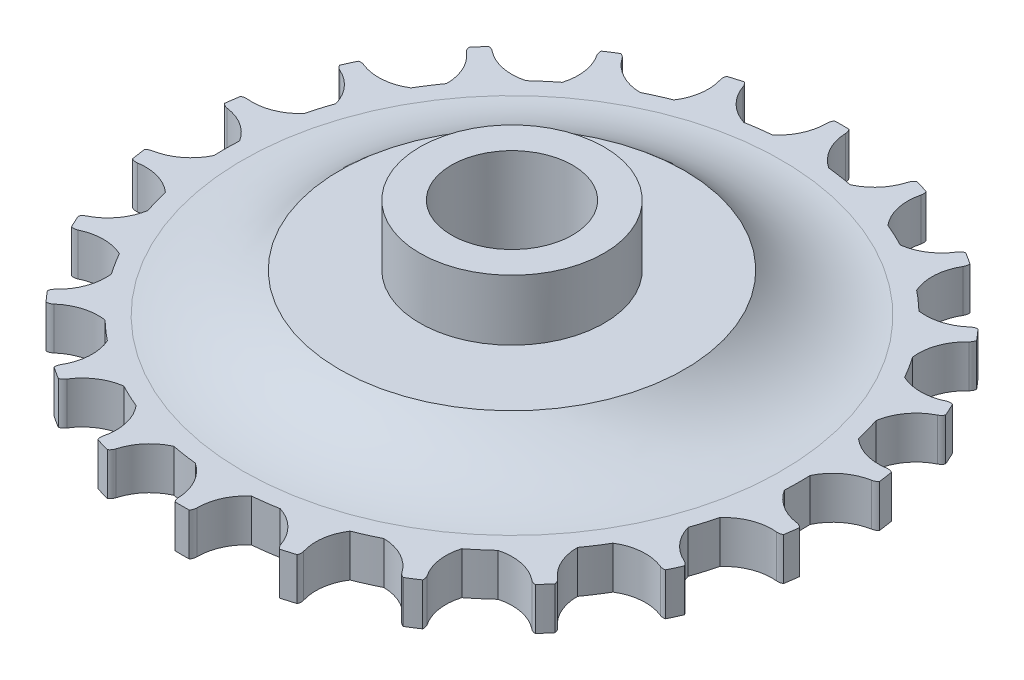
SolidWorks part; units mm, degrees
ref_plane "Front Plane" through (0, 0, 0) normal (0, 0, 1) x (1, 0, 0)
ref_plane "Top Plane" through (0, 0, 0) normal (0, 1, 0) x (1, 0, 0)
ref_plane "Right Plane" through (0, 0, 0) normal (1, 0, 0) x (0, 0, -1)
other "Configuration Table"
sketch "Sketch1" plane through (0, 0, 0) normal (0, 1, 0) x (1, 0, 0)
  line L0 (0, 55) -> (0, 0) construction
  line L1 (-7.2581, 50.4809) -> (0, 0) construction
  line L2 (0, 0) -> (7.2581, 50.4809) construction
  line L3 (-7.2581, 50.4809) -> (7.2581, 50.4809) construction
  circle A62 centre (0, 0) radius 10
  circle A64 centre (0, 0) radius 47.5 construction
  arc A65 (1.4988, 53.5593) -> (-1.4999, 53.4811) centre (0, 53.5) ccw
  arc A66 (-1.4999, 53.4811) -> (-4.294, 47.3055) centre (-9.4992, 53.3805) cw
  arc A67 (1.4988, 53.5593) -> (5.0355, 47.2323) centre (9.4926, 53.8757) ccw
  arc A68 (13.6282, 51.7373) -> (9.2075, 46.5991) centre (5.9246, 53.8944) cw
  arc A69 (16.5275, 50.9675) -> (13.6282, 51.7373) centre (15.0727, 51.3329) ccw
  arc A70 (16.5275, 50.9675) -> (18.1384, 43.9004) centre (24.2866, 49.019) ccw
  arc A71 (27.6523, 45.8021) -> (21.963, 42.1174) centre (20.8684, 50.0422) cw
  arc A72 (30.2172, 44.2466) -> (27.6523, 45.8021) centre (28.9243, 45.0071) ccw
  arc A73 (30.2172, 44.2466) -> (29.7718, 37.012) centre (37.1131, 40.1911) ccw
  arc A74 (39.4361, 36.1562) -> (32.9392, 34.2237) centre (34.1216, 42.1358) cw
  arc A75 (41.459, 33.9412) -> (39.4361, 36.1562) centre (40.4326, 35.035) ccw
  arc A76 (41.459, 33.9412) -> (38.9934, 27.125) centre (46.9329, 28.1071) ccw
  arc A77 (48.0251, 23.5812) -> (41.2468, 23.5574) centre (44.6105, 30.8159) cw
  arc A78 (49.3419, 20.886) -> (48.0251, 23.5812) centre (48.6653, 22.2247) ccw
  arc A79 (49.3419, 20.886) -> (45.0559, 15.0406) centre (52.9504, 13.746) ccw
  arc A80 (52.7233, 9.0958) -> (46.2129, 10.9826) centre (51.4853, 16.9994) cw
  arc A81 (53.2275, 6.1387) -> (52.7233, 9.0958) centre (52.9554, 7.6138) ccw
  arc A82 (53.2275, 6.1387) -> (47.4682, 1.7376) centre (54.6783, -1.7286) ccw
  arc A83 (53.1502, -6.1265) -> (47.4351, -2.482) centre (54.189, 1.8057) cw
  arc A84 (52.8009, -9.1059) -> (53.1502, -6.1265) centre (52.9554, -7.6138) ccw
  arc A85 (52.8009, -9.1059) -> (46.035, -11.7061) centre (51.9764, -17.0633) ccw
  arc A86 (49.2712, -20.8525) -> (44.8144, -15.7455) centre (52.5027, -13.5342) cw
  arc A87 (48.0966, -23.6127) -> (49.2712, -20.8525) centre (48.6653, -22.2247) ccw
  arc A88 (48.0966, -23.6127) -> (40.8722, -24.2015) centre (45.0637, -31.0155) ccw
  arc A89 (41.4006, -33.8892) -> (38.5631, -27.7333) centre (46.563, -27.7777) cw
  arc A90 (39.4959, -36.2066) -> (41.4006, -33.8892) centre (40.4326, -35.035) ccw
  arc A91 (39.4959, -36.2066) -> (32.3983, -34.7362) centre (34.5002, -42.4551) ccw
  arc A92 (30.1759, -44.1803) -> (29.1876, -37.4744) centre (36.8509, -39.7708) cw
  arc A93 (27.6955, -45.8673) -> (30.1759, -44.1803) centre (28.9243, -45.0071) ccw
  arc A94 (27.6955, -45.8673) -> (21.2996, -42.4568) centre (21.1418, -50.4552) ccw
  arc A95 (16.5065, -50.8922) -> (17.4475, -44.1796) centre (24.1535, -48.5419) cw
  arc A96 (13.6513, -51.8121) -> (16.5065, -50.8922) centre (15.0727, -51.3329) ccw
  arc A97 (13.6513, -51.8121) -> (8.4754, -46.7378) centre (6.0705, -54.3677) ccw
  arc A98 (1.4999, -53.4811) -> (4.294, -47.3055) centre (9.4992, -53.3805) cw
  arc A99 (-1.4988, -53.5593) -> (1.4999, -53.4811) centre (0, -53.5) ccw
  arc A100 (-1.4988, -53.5593) -> (-5.0355, -47.2323) centre (-9.4926, -53.8757) ccw
  arc A101 (-13.6282, -51.7373) -> (-9.2075, -46.5991) centre (-5.9246, -53.8944) cw
  arc A102 (-16.5275, -50.9675) -> (-13.6282, -51.7373) centre (-15.0727, -51.3329) ccw
  arc A103 (-16.5275, -50.9675) -> (-18.1384, -43.9004) centre (-24.2866, -49.019) ccw
  arc A104 (-27.6523, -45.8021) -> (-21.963, -42.1174) centre (-20.8684, -50.0422) cw
  arc A105 (-30.2172, -44.2466) -> (-27.6523, -45.8021) centre (-28.9243, -45.0071) ccw
  arc A106 (-30.2172, -44.2466) -> (-29.7718, -37.012) centre (-37.1131, -40.1911) ccw
  arc A107 (-39.4361, -36.1562) -> (-32.9392, -34.2237) centre (-34.1216, -42.1358) cw
  arc A108 (-41.459, -33.9412) -> (-39.4361, -36.1562) centre (-40.4326, -35.035) ccw
  arc A109 (-41.459, -33.9412) -> (-38.9934, -27.125) centre (-46.9329, -28.1071) ccw
  arc A110 (-48.0251, -23.5812) -> (-41.2468, -23.5574) centre (-44.6105, -30.8159) cw
  arc A111 (-49.3419, -20.886) -> (-48.0251, -23.5812) centre (-48.6653, -22.2247) ccw
  arc A112 (-49.3419, -20.886) -> (-45.0559, -15.0406) centre (-52.9504, -13.746) ccw
  arc A113 (-52.7233, -9.0958) -> (-46.2129, -10.9826) centre (-51.4853, -16.9994) cw
  arc A114 (-53.2275, -6.1387) -> (-52.7233, -9.0958) centre (-52.9554, -7.6138) ccw
  arc A115 (-53.2275, -6.1387) -> (-47.4682, -1.7376) centre (-54.6783, 1.7286) ccw
  arc A116 (-53.1502, 6.1265) -> (-47.4351, 2.482) centre (-54.189, -1.8057) cw
  arc A117 (-52.8009, 9.1059) -> (-53.1502, 6.1265) centre (-52.9554, 7.6138) ccw
  arc A118 (-52.8009, 9.1059) -> (-46.035, 11.7061) centre (-51.9764, 17.0633) ccw
  arc A119 (-49.2712, 20.8525) -> (-44.8144, 15.7455) centre (-52.5027, 13.5342) cw
  arc A120 (-48.0966, 23.6127) -> (-49.2712, 20.8525) centre (-48.6653, 22.2247) ccw
  arc A121 (-48.0966, 23.6127) -> (-40.8722, 24.2015) centre (-45.0637, 31.0155) ccw
  arc A122 (-41.4006, 33.8892) -> (-38.5631, 27.7333) centre (-46.563, 27.7777) cw
  arc A123 (-39.4959, 36.2066) -> (-41.4006, 33.8892) centre (-40.4326, 35.035) ccw
  arc A124 (-39.4959, 36.2066) -> (-32.3983, 34.7362) centre (-34.5002, 42.4551) ccw
  arc A125 (-30.1759, 44.1803) -> (-29.1876, 37.4744) centre (-36.8509, 39.7708) cw
  arc A126 (-27.6955, 45.8673) -> (-30.1759, 44.1803) centre (-28.9243, 45.0071) ccw
  arc A127 (-27.6955, 45.8673) -> (-21.2996, 42.4568) centre (-21.1418, 50.4552) ccw
  arc A128 (-16.5065, 50.8922) -> (-17.4475, 44.1796) centre (-24.1535, 48.5419) cw
  arc A129 (-13.6513, 51.8121) -> (-16.5065, 50.8922) centre (-15.0727, 51.3329) ccw
  arc A130 (-13.6513, 51.8121) -> (-8.4754, 46.7378) centre (-6.0705, 54.3677) ccw
  arc A131 (-32.3983, 34.7362) -> (-29.1876, 37.4744) centre (0, 0) cw
  arc A132 (-21.2996, 42.4568) -> (-17.4475, 44.1796) centre (0, 0) cw
  arc A133 (-8.4754, 46.7378) -> (-4.294, 47.3055) centre (0, 0) cw
  arc A134 (5.0355, 47.2323) -> (9.2075, 46.5991) centre (0, 0) cw
  arc A135 (18.1384, 43.9004) -> (21.963, 42.1174) centre (0, 0) cw
  arc A136 (29.7718, 37.012) -> (32.9392, 34.2237) centre (0, 0) cw
  arc A137 (38.9934, 27.125) -> (41.2468, 23.5574) centre (0, 0) cw
  arc A138 (45.0559, 15.0406) -> (46.2129, 10.9826) centre (0, 0) cw
  arc A139 (47.4682, 1.7376) -> (47.4351, -2.482) centre (0, 0) cw
  arc A140 (46.035, -11.7061) -> (44.8144, -15.7455) centre (0, 0) cw
  arc A141 (40.8722, -24.2015) -> (38.5631, -27.7333) centre (0, 0) cw
  arc A142 (32.3983, -34.7362) -> (29.1876, -37.4744) centre (0, 0) cw
  arc A143 (21.2996, -42.4568) -> (17.4475, -44.1796) centre (0, 0) cw
  arc A144 (8.4754, -46.7378) -> (4.294, -47.3055) centre (0, 0) cw
  arc A145 (-5.0355, -47.2323) -> (-9.2075, -46.5991) centre (0, 0) cw
  arc A146 (-18.1384, -43.9004) -> (-21.963, -42.1174) centre (0, 0) cw
  arc A147 (-29.7718, -37.012) -> (-32.9392, -34.2237) centre (0, 0) cw
  arc A148 (-38.9934, -27.125) -> (-41.2468, -23.5574) centre (0, 0) cw
  arc A149 (-45.0559, -15.0406) -> (-46.2129, -10.9826) centre (0, 0) cw
  arc A150 (-47.4682, -1.7376) -> (-47.4351, 2.482) centre (0, 0) cw
  arc A151 (-46.035, 11.7061) -> (-44.8144, 15.7455) centre (0, 0) cw
  arc A152 (-40.8722, 24.2015) -> (-38.5631, 27.7333) centre (0, 0) cw
  circle A153 centre (0, 0) radius 51 construction
  point P3 (0, 51)
  point P225 (0, 0)
  dimension "D1" = 20
  dimension "D2" = 51
  dimension "D3" = 95
  dimension "D4" = 3
  dimension "D5" = 8
  dimension "D6" = 8
  dimension "D7" = 8.182
  dimension "D8" = 8.182
  dimension "D9" = 14.5161
extrude "Boss-Extrude1" add sketch "Sketch1" along normal blind 20
sketch "Sketch4" plane through (0, 20, 0) normal (0, 1, 0) x (1, 0, 0)
  circle A0 centre (0, 0) radius 10
  circle A1 centre (0, 0) radius 15.2026
extrude "Boss-Extrude4" add sketch "Sketch4" along normal blind 10
ref_plane "Plane1" through (0, 0, -55) normal (0, 0, -1) x (-1, 0, 0)
ref_axis "Axis1" through (0, 30, 0) along (0, -1, 0)
sketch "Sketch6" plane through (0, 0, 0) normal (0, 0, 1) x (1, 0, 0)
  line L0 (-54.4554, 20) -> (-54.4554, 0) construction
  line L1 (-54.4554, 13.5) -> (-54.4554, 6.5)
  line L2 (-54.4554, 13.5) -> (-44.4554, 13.5)
  line L3 (-54.4554, 6.5) -> (-44.4554, 6.5)
  line L4 (-21.963, 20) -> (-27.6523, 20) construction
  line L5 (-27.6523, 0) -> (-21.963, 0) construction
  line L6 (-28.4554, 20) -> (-62.6958, 20)
  line L7 (-62.6958, 20) -> (-62.6958, 0)
  line L8 (-62.6958, 0) -> (-28.4554, 0)
  arc A0 (-44.4554, 13.5) -> (-28.4554, 20) centre (-44.4554, 36.4423) ccw
  arc A1 (-44.4554, 6.5) -> (-28.4554, 0) centre (-44.4554, -16.4423) cw
  point P0 (-54.4554, 10)
  point P6 (-54.4554, 10)
  dimension "D1" = 7
  dimension "D2" = 10
  dimension "D3" = 10
  dimension "D4" = 16
  dimension "D5" = 16
revolve "Cut-Revolve1" cut sketch "Sketch6" angle 360 about axis through (0, 30, 0) along (0, -1, 0)
sketch "Sketch7" plane through (0, 0, 0) normal (0, -1, 0) x (1, 0, 0)
  circle A0 centre (0, 0) radius 10
  circle A1 centre (0, 0) radius 19.9177
extrude "Boss-Extrude5" add sketch "Sketch7" along normal blind 3
